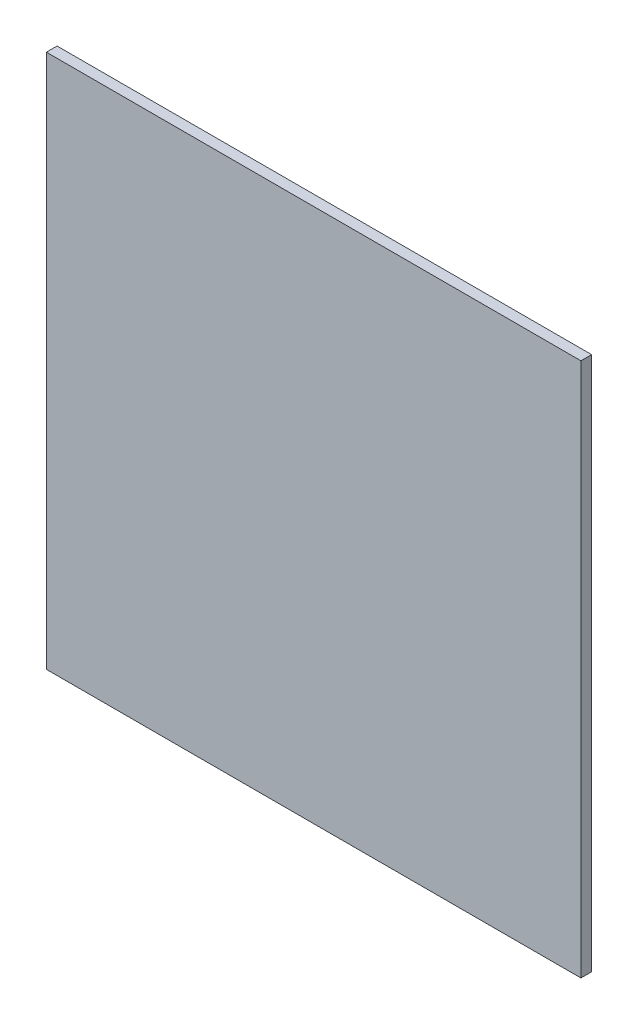
SolidWorks part; units mm, degrees
ref_plane "Front Plane" through (0, 0, 0) normal (0, 0, 1) x (1, 0, 0)
ref_plane "Top Plane" through (0, 0, 0) normal (0, 1, 0) x (1, 0, 0)
ref_plane "Right Plane" through (0, 0, 0) normal (1, 0, 0) x (0, 0, -1)
other "Configuration Table"
sketch "Sketch1" plane through (0, 0, 0) normal (0, 0, 1) x (1, 0, 0)
  line L1 (-25, -25) -> (25, -25)
  line L2 (-25, -25) -> (-25, 25)
  line L3 (-25, 25) -> (25, 25)
  line L4 (25, -25) -> (25, 25)
  line L5 (-25, -25) -> (25, 25) construction
  line L6 (-25, 25) -> (25, -25) construction
  point P0 (0, 0)
  dimension "D1" = 50
  dimension "D2" = 50
extrude "Boss-Extrude1" add sketch "Sketch1" along normal blind 1
